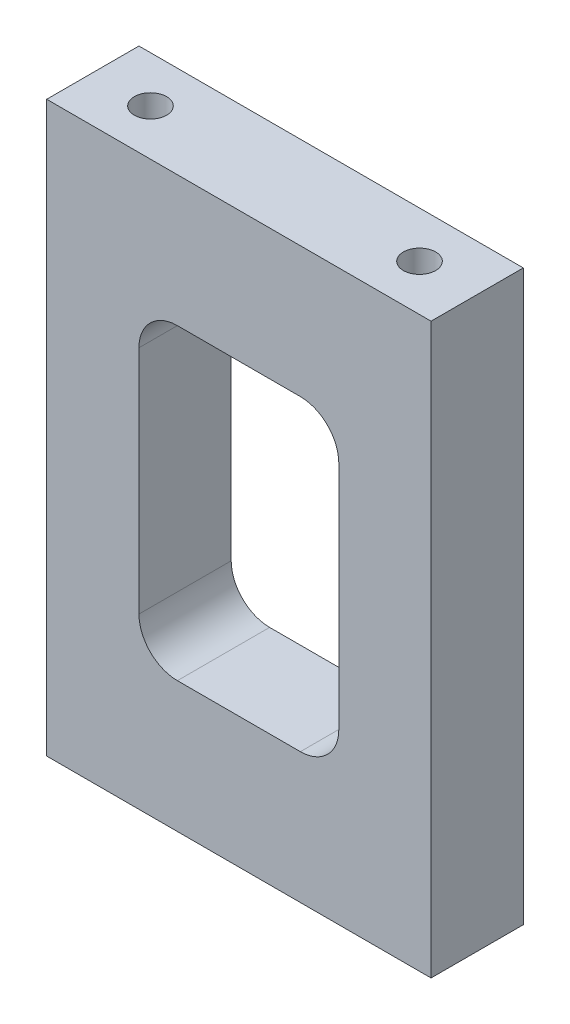
from build123d import *

# Parameters (mm, degrees)
SKETCH_1_W                  = 50
SKETCH_1_H                  = 74
EXTRUDE_1_DEPTH             = 6
HOLE_WIZARD_M5_1_AT_2_COUNT = 2
HOLE_WIZARD_M5_1_AT_2_PITCH = 35
CUT_EXTRUDE_1_DEPTH         = 47.238512087


with BuildPart() as part:
    # 草图1 → 凸台-拉伸1 (new, symmetric)
    with BuildSketch(Plane.XY):
        Rectangle(SKETCH_1_W, SKETCH_1_H)
    extrude(amount=EXTRUDE_1_DEPTH, both=True)

    # 草图3 → M5 螺纹孔1 (revolve, cut)
    with BuildSketch(Plane(origin=(-17.5, -37, 0), x_dir=(0, 0, -1), z_dir=(1, 0, 0))):
        Polygon((0, 0), (0, 13.6618073), (2.1, 12.4), (2.1, 0), align=None)
    hole_wizard_m5_1 = revolve(axis=Axis((-17.5, -43.35, 0), (0, 1, 0)), mode=Mode.SUBTRACT)

    # M5 螺纹孔1 at 2: M5 螺纹孔1 ×2
    with Locations(*[(i * HOLE_WIZARD_M5_1_AT_2_PITCH, 0, 0) for i in range(1, HOLE_WIZARD_M5_1_AT_2_COUNT)]):
        add(hole_wizard_m5_1, mode=Mode.SUBTRACT)

    # 镜向1: M5 螺纹孔1 across plane
    add(hole_wizard_m5_1.mirror(Plane.ZX), mode=Mode.SUBTRACT)

    # 镜向1 copy 1 sketch → 镜向1 copy 1 (revolve, cut)
    with BuildSketch(Plane(origin=(17.5, 37, 0), x_dir=(0, 0, -1), z_dir=(1, 0, 0))):
        Polygon((0, 0), (0, -13.6618073), (2.1, -12.4), (2.1, 0), align=None)
    revolve(axis=Axis((17.5, 43.35, 0), (0, 1, 0)), mode=Mode.SUBTRACT)

    # 草图5 → 切除-拉伸1 (cut, through all)
    with BuildSketch(Plane.XY.offset(6)):
        with BuildLine():
            Line((-8, -20), (8, -20))
            ThreePointArc((8, -20), (11.535533906, -18.535533906), (13, -15))
            Line((13, -15), (13, 15))
            ThreePointArc((13, 15), (11.535533906, 18.535533906), (8, 20))
            Line((8, 20), (-8, 20))
            ThreePointArc((-8, 20), (-11.535533906, 18.535533906), (-13, 15))
            Line((-13, 15), (-13, -15))
            ThreePointArc((-13, -15), (-11.535533906, -18.535533906), (-8, -20))
        make_face()
    extrude(amount=-CUT_EXTRUDE_1_DEPTH, mode=Mode.SUBTRACT)


solid = part.part
